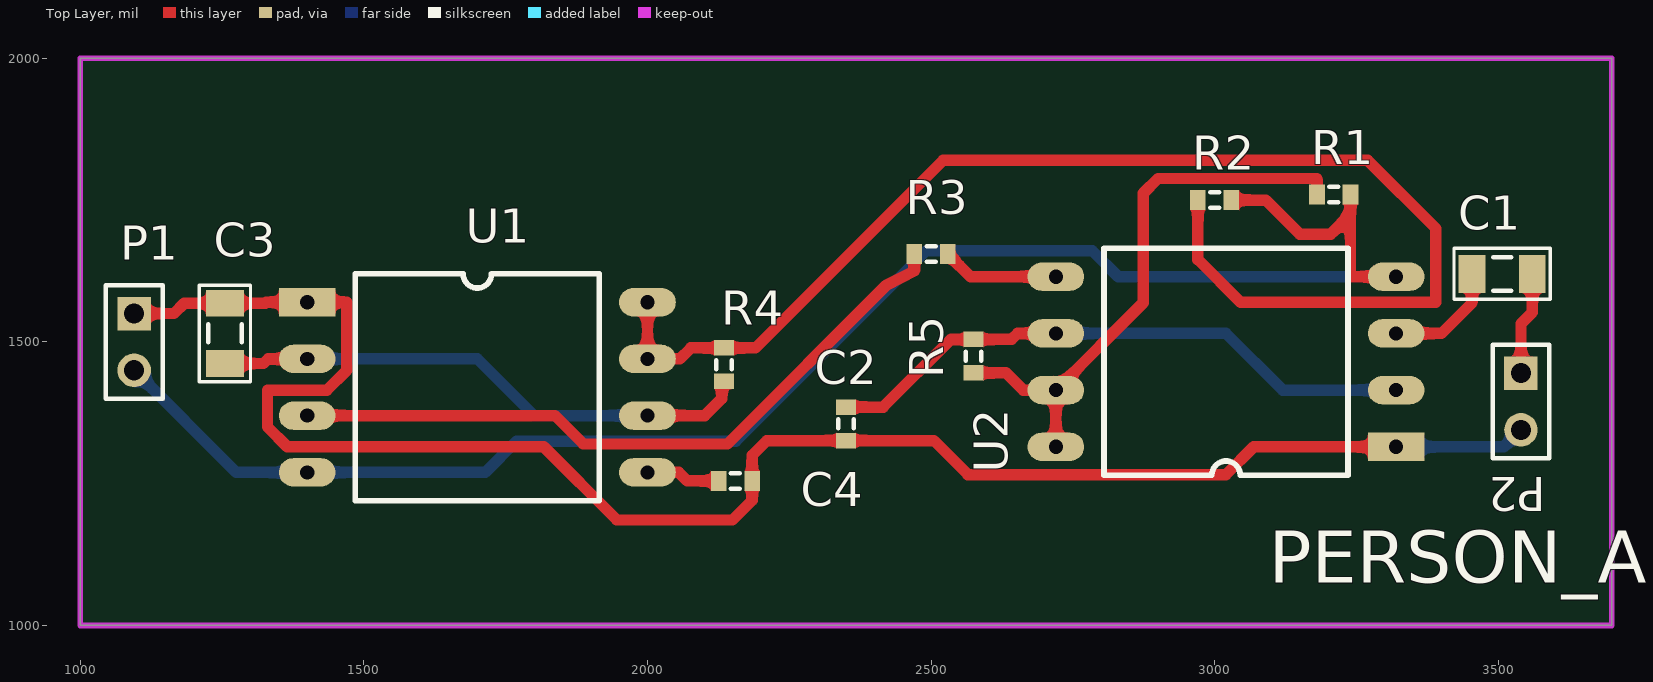
[diagram p0: Top Layer view]
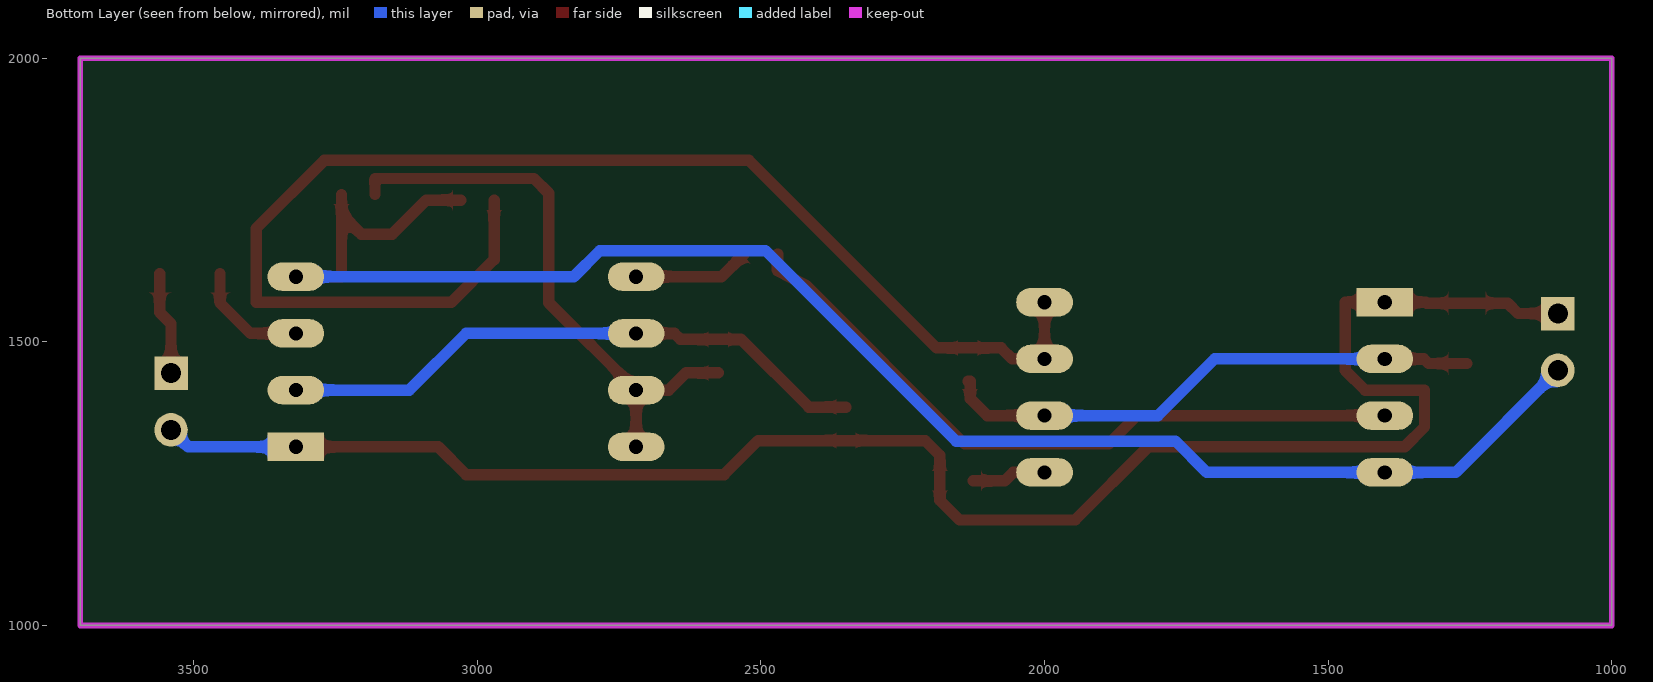
[diagram p1: Bottom Layer view, seen from below]
# Altium PCB MISC89130.PcbDoc
Units mil, origin at the board's own origin, x right, y up, seen from the top; angles counter-clockwise.
Board outline 2700 x 1000 mil, 2 copper layers (Top Layer, Bottom Layer); 13 components, 11 nets, 38 pads, 0 vias.

## Layer stack, top to bottom (the 12.6 mil dielectric is the usual default, probably not edited)
Top Solder: solder mask 0.4, Solder Resist, Dk 3.5
Top Layer: signal copper 1.4
Dielectric 1: dielectric 12.6, FR-4, Dk 4.8
Bottom Layer: signal copper 1.4
Bottom Solder: solder mask 0.4, Solder Resist, Dk 3.5

## Board outline
1000,1000 1000,2000 3700,2000 3700,1000

## Design rules (kind name [scope] priority, off if disabled: settings)
Clearance [All] p1: gap=10
HoleSize [All] p1: absolutevalues=TRUE maxlimit=7777 minlimit=1 maxpercent=80.000 minpercent=20.000
MinimumSolderMaskSliver [All] p1: minsoldermaskwidth=0
PolygonConnect [All] p1: connectstyle=Relief reliefconductorwidth=10 reliefentries=4 polygonreliefangle="90 Angle" airgapwidth=10
RoutingVias [All] p1: holewidth=28 width=50 viastyle="Through Hole" minholewidth=28 minwidth=50 maxholewidth=28 maxwidth=50
SilkToSilkClearance [All] p1: silktosilkclearance=0
SilkToSolderMaskClearance [IsPad] p1: minsilkscreentomaskgap=0 clearancetoexposedcopper=TRUE
SolderMaskExpansion [All] p1: expansion=4
Width [All] p1: maxlimit=20 minlimit=20 preferedwidth=20
26 further rules are at their usual default settings.

## Components (designator, comment, footprint, x,y, rotation, side; value= is the part's Value field where it differs from the comment)
C1 "10UF" C1206 3506.85,1620 r0 top
C2 "Cap" J1-0603 2350,1355.47 r90 top
C3 "10UF" C1206 1255,1515 r90 top
C4 "Cap" J1-0603 2155,1255 r180 top
P1 "Header 2" HDR1X2 1095,1550 r270 top
P2 "Header 2" HDR1X2 3540,1445 r270 top
R1 "10K" J1-0603 3210,1760 r0 top
R2 "10K" J1-0603 3000,1750 r0 top
R3 "10K" J1-0603 2500,1655 r180 top
R4 "75K" J1-0603 2135,1460 r270 top
R5 "220K" J1-0603 2575,1475 r90 top
U1 "NE555" DIP8 1400,1570 r0 top
U2 "NE555" DIP8 3320,1315 r180 top

## Footprints (in the part's own frame and the unit in brackets; to place one, negate y for a bottom-side part, rotate by r counter-clockwise, add the part's x,y. Pads: shape width x height; smd on the part's side, far side on the other; paste and mask are expansions set on the pad)
C1206 [mm]
  rect 1.2x1.7 smd: 1(-1.35,0) 2(1.35,0)
  silkscreen extent -2.16,-1.14 2.16,1.14, body extent -1.7,-0.9 1.7,0.9, height 1.3
DIP8 [mil]
  rect 100x50 hole 25: 1(0,0)
  oval 100x50 hole 25: 2(0,-100) 3(0,-200) 4(0,-300) 5(600,-300) 6(600,-200) 7(600,-100) 8(600,0)
  silkscreen extent 85,-350 515,50
HDR1X2 [mm] "Connector; Header; 2 Position"
  rect 1.5x1.5 hole 0.9: 1(0,0)
  round 1.5 hole 0.9: 2(2.54,0)
  silkscreen extent -1.27,-1.27 3.81,1.27
J1-0603 [mm] "Chip Resistor, Body 1.6x0.8mm, IPC High Density"
  rect 0.7x0.9 smd: 1(-0.75,0) 2(0.75,0)
  silkscreen extent -0.2,-0.35 0.2,0.35, body extent -0.85,-0.48 0.85,0.48, height 0.9

## Part data
C1 C3: library part "Cap Pol3", "Polarized Capacitor (Surface Mount)"
C2 C4: "Capacitor"
P1 P2: "Header, 2-Pin"
R1 R2 R3 R4 R5: library part Res3, "Resistor"

## Nets (pads, with @x,y where several pads share a name; then routed paths per layer and width w, separated by ;. In a path a pad name is that pad's centre, name@x,y a point inside that pad or via, vN(x,y) a via of type N, cw(c..) or ccw(c..) an arc to the next point about the centre after c; other vN are vias at no path point)
GND: C2.1 C3.2 C4.1 P1.1 P2.2 U1.1 U2.1 | length 3162.8
  Top Layer w20: P1.1 1165,1550 1183.15,1568.15 C3.2 1326,1568.15 1327.85,1570 U1.1 1470,1570 1470,1450 1435,1415 1330,1415 1330,1350 1365,1315 1817,1315 1946,1186 2150,1186 2184.53,1220.53 C4.1 2184.53,1300 2210.47,1325.94 C2.1 2505,1325.94 2564.94,1266 3020,1266 3069,1315 U2.1
  Bottom Layer w20: U2.1 3510,1315 P2.2
NetC1_1: C1.1 U2.3 | length 207.2
  Top Layer w20: U2.3 3400,1515 3453.7,1568.7 C1.1
NetC1_2: C1.2 P2.1 | length 183.3
  Top Layer w20: P2.1 3540,1532 3560,1552 C1.2
NetC2_2: C2.2 R5.2 U2.2 U2.6 | length 1065.3
  Top Layer w20: C2.2 2415.47,1385 2535,1504.53 R5.2 2642,1504.53 2652.47,1515 U2.6
  Bottom Layer w20: U2.6 3020,1515 3120,1415 U2.2
NetC3_1: C3.1 R4.2 U1.2 U1.6 | length 967.7
  Top Layer w20: C3.1 1323,1461.85 1331.15,1470 U1.2 ; U1.6 2101,1370 2131,1400 2131,1430.47 R4.2
  Bottom Layer w20: U1.2 1700,1470 1800,1370 U1.6
NetC4_2: C4.2 U1.5 | length 131.7
  Top Layer w20: U1.5 2055,1270 2070,1255 C4.2
NetR1_1: R1.1 R5.1 U2.7 U2.8 | length 1013.7
  Top Layer w20: R5.1 2632,1445.47 2662.47,1415 U2.7 ; U2.8 U2.7 ; R1.1 3180.47,1788 2900,1788 2874,1762 2874,1569 U2.7
NetR2_1: R2.1 R4.1 U1.7 U1.8 | length 2370.3
  Top Layer w20: U1.8 U1.7 2057,1470 2076.53,1489.53 R4.1 2190.53,1489.53 2521,1820 3270,1820 3390,1700 3390,1570 3045.47,1570 2970.47,1645 R2.1
NetR3_1: R3.1 U2.5 | length 207
  Top Layer w20: R3.1 2569.53,1615 U2.5
NetR3_2: R3.2 U1.3 | length 1243.1
  Top Layer w20: U1.3 1837,1370 1887,1320 2141,1320 2421,1600 2470.47,1625 R3.2
VCC: P1.2 R1.2 R2.2 U1.4 U2.4 | length 2955.4
  Top Layer w20: R2.2 3090,1750 3150,1690 3204.53,1690 3239.53,1725 ; R1.2 3239.53,1725 ; U2.4 3239.53,1615 3239.53,1725
  Bottom Layer w20: P1.2 1275,1270 U1.4 1714,1270 1769,1325 2156,1325 2492,1661 2784,1661 2830,1615 U2.4

## Keep-outs
Keep-Out Layer:
  the board outline again, w10

## Silkscreen, mask and mechanical layers (free items; w line width, h text height)
Top Overlay:
  text "PERSON_A" at 3095,1045 h157.48